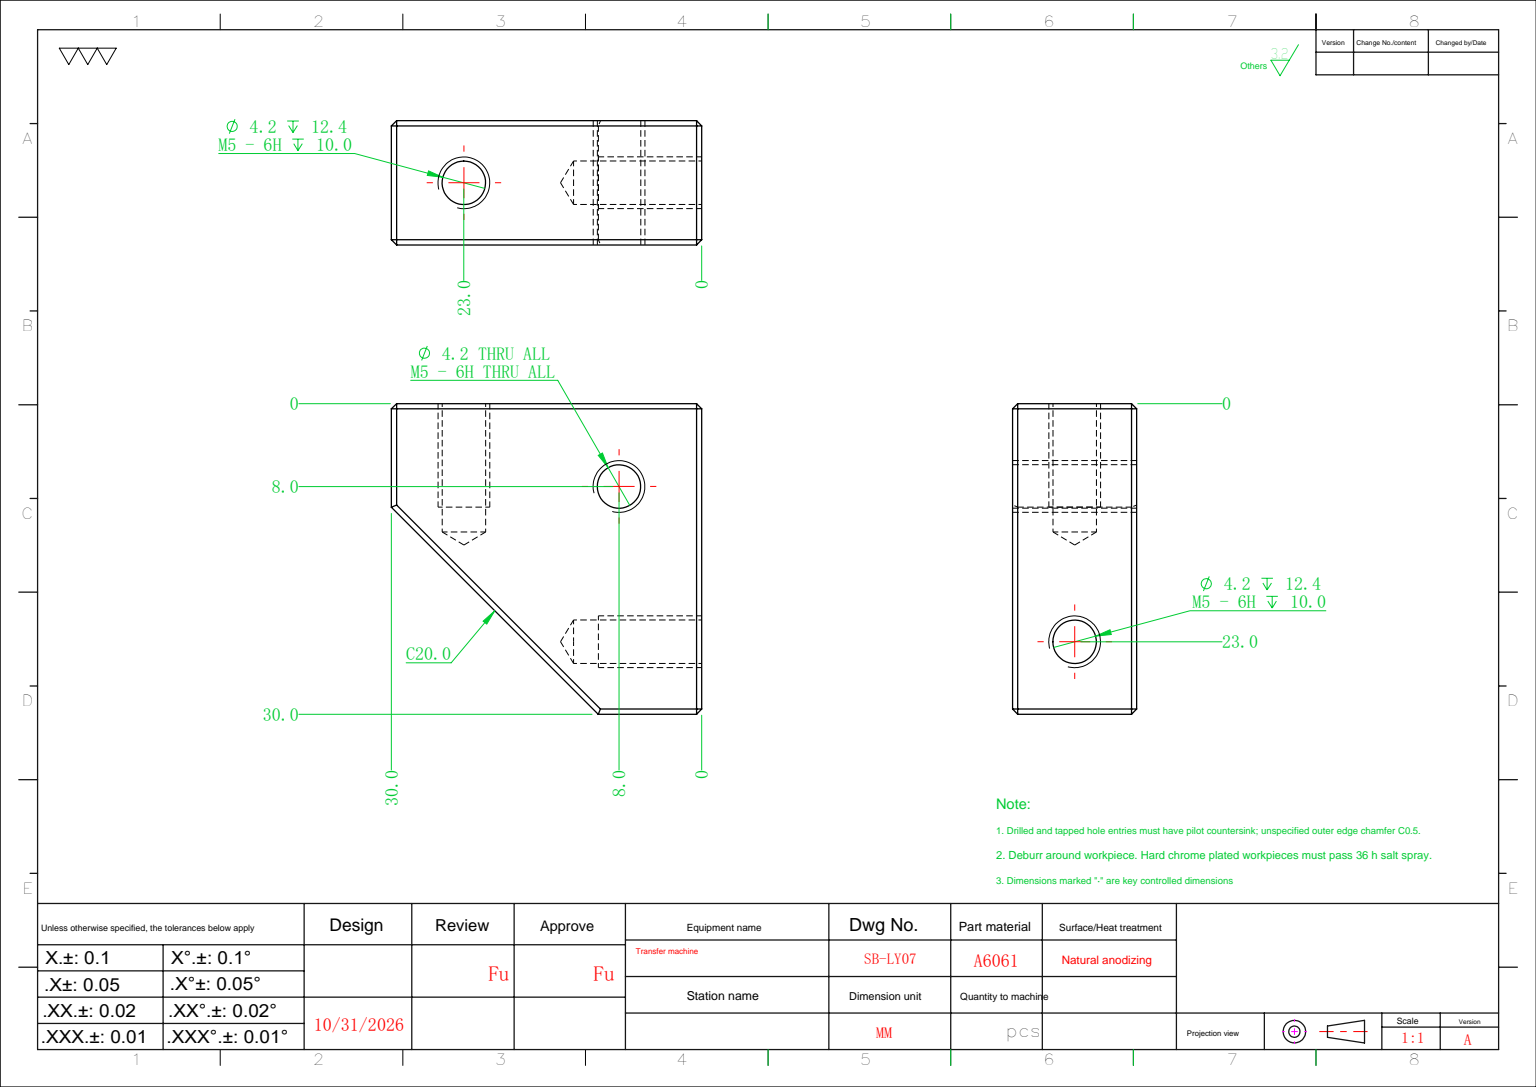
SolidWorks part; units mm, degrees
ref_plane "前视基准面" through (0, 0, 0) normal (0, 0, 1) x (1, 0, 0)
ref_plane "上视基准面" through (0, 0, 0) normal (0, 1, 0) x (1, 0, 0)
ref_plane "右视基准面" through (0, 0, 0) normal (1, 0, 0) x (0, 0, -1)
sketch "草图1" plane through (0, 0, 0) normal (0, 0, 1) x (1, 0, 0)
  line L1 (-15, -15) -> (15, -15)
  line L2 (-15, -15) -> (-15, 15)
  line L3 (-15, 15) -> (15, 15)
  line L4 (15, -15) -> (15, 15)
  line L5 (-15, -15) -> (15, 15) construction
  line L6 (-15, 15) -> (15, -15) construction
  point P0 (0, 0)
  dimension "D1" = 30
  dimension "D2" = 30
extrude "凸台-拉伸1" add sketch "草图1" along normal blind 12
chamfer "倒角1" distance 20 angle 45 1 edges at (15, 15, 6)
hole_wizard "M5 螺纹孔1" positions "草图2" profile "草图3" tap size "M5" standard "ISO" end condition through all
sketch "草图2" plane through (0, 0, 12) normal (0, 0, 1) x (1, 0, 0)
  line L0 (-15, 15) -> (-15, -15) construction
  line L1 (-15, -15) -> (15, -15) construction
  point P0 (-7, -7)
  dimension "D1" = 8
  dimension "D2" = 8
sketch "草图3" plane through (-7, -7, 12) normal (1, 0, 0) x (0, -1, 0)
  line L0 (0, 0) -> (0, 12)
  line L1 (0, 12) -> (2.1, 12)
  line L2 (2.1, 12) -> (2.1, 0)
  line L5 (2.1, 0) -> (0, 0)
  line L11 (0, -6.35) -> (0, 107.95) construction
  dimension "通孔螺纹孔钻头直径" = 4.2
  dimension "通孔螺纹孔钻头深度" = 12
cosmetic thread "孔螺蚊线1" parameters "D2"=5
hole_wizard "M5 螺纹孔2" positions "草图4" profile "草图5" tap size "M5" standard "ISO"
sketch "草图4" plane through (0, -15, 0) normal (0, -1, 0) x (-1, 0, 0)
  line L0 (15, -6) -> (-15, -6) construction
  line L1 (15, -12) -> (15, 0) construction
  line L2 (-15, -12) -> (-15, 0) construction
  point P0 (-8, -6)
  dimension "D1" = 23
sketch "草图5" plane through (8, -15, 6) normal (1, 0, 0) x (0, 0, -1)
  line L0 (0, 0) -> (0, 13.6618)
  line L1 (0, 13.6618) -> (2.1, 12.4)
  line L2 (2.1, 12.4) -> (2.1, 0)
  line L5 (2.1, 0) -> (0, 0)
  line L10 (0, 13.6618) -> (-2.1, 12.4) construction
  line L11 (0, -6.35) -> (0, 107.95) construction
  dimension "螺纹孔钻头直径" = 4.2
  dimension "螺纹孔钻头深度" = 12.4
  dimension "导头角度" = 118
cosmetic thread "孔螺蚊线2" parameters "D1"=10, "D2"=5
hole_wizard "M5 螺纹孔3" positions "草图6" profile "草图7" tap size "M5" standard "ISO"
sketch "草图6" plane through (-15, 0, 0) normal (-1, 0, 0) x (0, 0, 1)
  line L0 (6, -15) -> (6, 15) construction
  line L1 (12, -15) -> (0, -15) construction
  line L2 (12, 15) -> (0, 15) construction
  point P0 (6, 8)
  dimension "D1" = 23
sketch "草图7" plane through (-15, 8, 6) normal (0, 1, 0) x (0, 0, 1)
  line L0 (0, 0) -> (0, 13.6618)
  line L1 (0, 13.6618) -> (2.1, 12.4)
  line L2 (2.1, 12.4) -> (2.1, 0)
  line L5 (2.1, 0) -> (0, 0)
  line L10 (0, 13.6618) -> (-2.1, 12.4) construction
  line L11 (0, -6.35) -> (0, 107.95) construction
  dimension "螺纹孔钻头直径" = 4.2
  dimension "螺纹孔钻头深度" = 12.4
  dimension "导头角度" = 118
cosmetic thread "孔螺蚊线3" parameters "D1"=10, "D2"=5
chamfer "倒角2" distance 0.5 angle 45 13 edges at (15, -10, 0) (5, 5, 0) (-10, 15, 0) (-10, 15, 12) (5, 5, 12) (15, -10, 12) (0, -15, 12) (15, -15, 6) (0, -15, 0) (-15, 15, 6) (-15, 0, 12) (-15, -15, 6) (-15, 0, 0)
